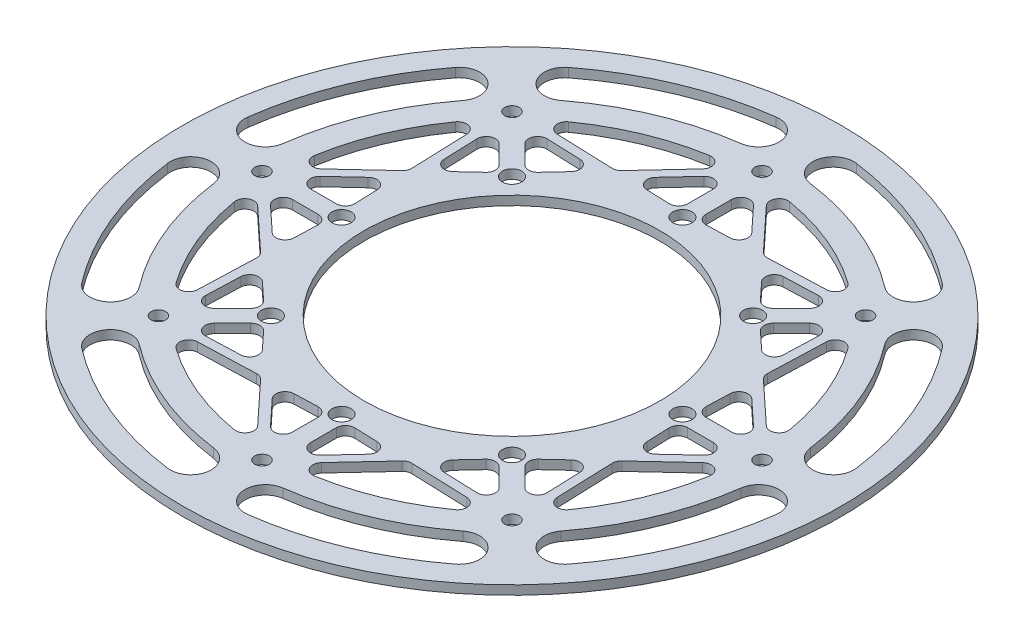
SolidWorks part; units mm, degrees
material "哈碳纤"
ref_plane "前视基准面" through (0, 0, 0) normal (0, 0, 1) x (1, 0, 0)
ref_plane "上视基准面" through (0, 0, 0) normal (0, 1, 0) x (1, 0, 0)
ref_plane "右视基准面" through (0, 0, 0) normal (1, 0, 0) x (0, 0, -1)
other "Configuration Table"
sketch "草图1" plane through (0, 0, 0) normal (0, 1, 0) x (1, 0, 0)
  line L0 (0, -1000) -> (0, 49000) construction
  line L1 (-38.352, 49.9813) -> (0, 0) construction
  line L2 (0, 0) -> (-8.2232, 62.461) construction
  line L3 (-24.1091, 58.2044) -> (0, 0) construction
  circle A0 centre (0, 0) radius 32.5
  circle A1 centre (0, 0) radius 72.5
  circle A2 centre (0, 0) radius 55 construction
  circle A3 centre (0, 55) radius 1.6
  circle A4 centre (38.8909, 38.8909) radius 1.6
  circle A5 centre (55, 0) radius 1.6
  circle A6 centre (38.8909, -38.8909) radius 1.6
  circle A7 centre (0, -55) radius 1.6
  circle A8 centre (-38.8909, -38.8909) radius 1.6
  circle A9 centre (-55, 0) radius 1.6
  circle A10 centre (-38.8909, 38.8909) radius 1.6
  circle A11 centre (0, 0) radius 37.5 construction
  circle A12 centre (0, 37.5) radius 2.1
  circle A13 centre (26.5165, 26.5165) radius 2.1
  circle A14 centre (37.5, 0) radius 2.1
  circle A15 centre (26.5165, -26.5165) radius 2.1
  circle A16 centre (0, -37.5) radius 2.1
  circle A17 centre (-26.5165, -26.5165) radius 2.1
  circle A18 centre (-37.5, 0) radius 2.1
  circle A19 centre (-26.5165, 26.5165) radius 2.1
  arc A20 (-38.352, 49.9813) -> (-8.2232, 62.461) centre (0, 0) cw construction
  arc A21 (-8.8105, 66.9225) -> (-41.0914, 53.5514) centre (0, 0) ccw
  arc A22 (-7.6358, 57.9995) -> (-35.6125, 46.4112) centre (0, 0) ccw
  arc A23 (-7.6358, 57.9995) -> (-8.8105, 66.9225) centre (-8.2232, 62.461) ccw
  arc A24 (-41.0914, 53.5514) -> (-35.6125, 46.4112) centre (-38.352, 49.9813) ccw
  arc A25 (8.2232, 62.461) -> (38.352, 49.9813) centre (0, 0) cw construction
  arc A26 (41.0914, 53.5514) -> (8.8105, 66.9225) centre (0, 0) ccw
  arc A27 (35.6125, 46.4112) -> (7.6358, 57.9995) centre (0, 0) ccw
  arc A28 (35.6125, 46.4112) -> (41.0914, 53.5514) centre (38.352, 49.9813) ccw
  arc A29 (8.8105, 66.9225) -> (7.6358, 57.9995) centre (8.2232, 62.461) ccw
  arc A30 (49.9813, 38.352) -> (62.461, 8.2232) centre (0, 0) cw construction
  arc A31 (66.9225, 8.8105) -> (53.5514, 41.0914) centre (0, 0) ccw
  arc A32 (57.9995, 7.6358) -> (46.4112, 35.6125) centre (0, 0) ccw
  arc A33 (57.9995, 7.6358) -> (66.9225, 8.8105) centre (62.461, 8.2232) ccw
  arc A34 (53.5514, 41.0914) -> (46.4112, 35.6125) centre (49.9813, 38.352) ccw
  arc A35 (62.461, -8.2232) -> (49.9813, -38.352) centre (0, 0) cw construction
  arc A36 (53.5514, -41.0914) -> (66.9225, -8.8105) centre (0, 0) ccw
  arc A37 (46.4112, -35.6125) -> (57.9995, -7.6358) centre (0, 0) ccw
  arc A38 (46.4112, -35.6125) -> (53.5514, -41.0914) centre (49.9813, -38.352) ccw
  arc A39 (66.9225, -8.8105) -> (57.9995, -7.6358) centre (62.461, -8.2232) ccw
  arc A40 (38.352, -49.9813) -> (8.2232, -62.461) centre (0, 0) cw construction
  arc A41 (8.8105, -66.9225) -> (41.0914, -53.5514) centre (0, 0) ccw
  arc A42 (7.6358, -57.9995) -> (35.6125, -46.4112) centre (0, 0) ccw
  arc A43 (7.6358, -57.9995) -> (8.8105, -66.9225) centre (8.2232, -62.461) ccw
  arc A44 (41.0914, -53.5514) -> (35.6125, -46.4112) centre (38.352, -49.9813) ccw
  arc A45 (-8.2232, -62.461) -> (-38.352, -49.9813) centre (0, 0) cw construction
  arc A46 (-41.0914, -53.5514) -> (-8.8105, -66.9225) centre (0, 0) ccw
  arc A47 (-35.6125, -46.4112) -> (-7.6358, -57.9995) centre (0, 0) ccw
  arc A48 (-35.6125, -46.4112) -> (-41.0914, -53.5514) centre (-38.352, -49.9813) ccw
  arc A49 (-8.8105, -66.9225) -> (-7.6358, -57.9995) centre (-8.2232, -62.461) ccw
  arc A50 (-49.9813, -38.352) -> (-62.461, -8.2232) centre (0, 0) cw construction
  arc A51 (-66.9225, -8.8105) -> (-53.5514, -41.0914) centre (0, 0) ccw
  arc A52 (-57.9995, -7.6358) -> (-46.4112, -35.6125) centre (0, 0) ccw
  arc A53 (-57.9995, -7.6358) -> (-66.9225, -8.8105) centre (-62.461, -8.2232) ccw
  arc A54 (-53.5514, -41.0914) -> (-46.4112, -35.6125) centre (-49.9813, -38.352) ccw
  arc A55 (-62.461, 8.2232) -> (-49.9813, 38.352) centre (0, 0) cw construction
  arc A56 (-53.5514, 41.0914) -> (-66.9225, 8.8105) centre (0, 0) ccw
  arc A57 (-46.4112, 35.6125) -> (-57.9995, 7.6358) centre (0, 0) ccw
  arc A58 (-46.4112, 35.6125) -> (-53.5514, 41.0914) centre (-49.9813, 38.352) ccw
  arc A59 (-66.9225, 8.8105) -> (-57.9995, 7.6358) centre (-62.461, 8.2232) ccw
  point P25 (0, 0)
  point P43 (0, 0)
  point P44 (-24.1091, 58.2044)
  point P56 (24.1091, 58.2044)
  point P63 (58.2044, 24.1091)
  point P70 (58.2044, -24.1091)
  point P77 (24.1091, -58.2044)
  point P84 (-24.1091, -58.2044)
  point P89 (0, 0)
  point P90 (-58.2044, -24.1091)
  point P97 (-58.2044, 24.1091)
  dimension "D1" = 65
  dimension "D2" = 145
  dimension "D3" = 110
  dimension "D4" = 3.2
  dimension "D6" = 75
  dimension "D7" = 4.2
  dimension "D9" = 9
  dimension "D10" = 63
  dimension "D11" = 30
  dimension "D13" = 22.5
  dimension "D5" = 8
  dimension "D8" = 8
  dimension "D12" = 8
extrude "凸台-拉伸1" add sketch "草图1" along normal blind 2
sketch "草图2" plane through (0, 2, 0) normal (0, 1, 0) x (1, 0, 0)
  line L0 (0, 55) -> (26.5165, 26.5165) construction
  line L1 (0, 37.5) -> (38.8909, 38.8909) construction
  line L2 (0, 55) -> (0, 37.5)
  line L3 (26.5165, 26.5165) -> (38.8909, 38.8909)
  line L4 (1.3824, 54.9826) -> (27.2241, 27.2241)
  line L5 (0, 38.5006) -> (37.9011, 39.8561)
  line L6 (0, 53.5324) -> (20.7675, 31.2244)
  line L7 (7.3941, 36.7638) -> (37.8531, 37.8531)
  line L8 (0.0357, 36.5006) -> (38.9266, 37.8915) construction
  line L9 (-0.7319, 54.3186) -> (25.7846, 25.8351) construction
  line L10 (-0.0357, 38.4994) -> (38.8551, 39.8902) construction
  line L11 (0.7319, 55.6814) -> (27.2484, 27.1979) construction
  line L12 (-1, 55) -> (-1, 37.5)
  line L13 (27.2236, 25.8094) -> (39.598, 38.1838)
  line L14 (2, 55) -> (2, 37.5)
  line L15 (25.1023, 27.9307) -> (37.4767, 40.3051)
  arc A0 (38.8909, 38.8909) -> (0, 55) centre (0, 0) ccw
  arc A1 (26.5165, 26.5165) -> (0, 37.5) centre (0, 0) ccw
  arc A2 (39.598, 39.598) -> (0, 56) centre (0, 0) ccw
  arc A3 (37.4767, 37.4767) -> (0, 53) centre (0, 0) ccw
  circle M13 centre (0, 37.5) radius 2.1
  circle M17 centre (26.5165, 26.5165) radius 2.1
  dimension "D1" = 1
  dimension "D2" = 1
  dimension "D3" = 1
  dimension "D4" = 2
  dimension "D5" = 1
  dimension "D6" = 2
extrude "切除-拉伸1" cut sketch "草图2" against normal through all both and the other way through all contours L6 L14 L5 M13 | L5 A3 L4 | L15 L7 L4 M17
fillet "圆角1" radius 2 9 edges at (13.5428, 1, -38.985) (2, 1, -38.5722) (3.3254, 1, -52.8956) (35.0514, 1, -39.7542) (16.1873, 1, -39.0796) (34.9198, 1, -37.7482) (25.8604, 1, -28.6889) (17.9903, 1, -37.1428) (2, 1, -51.384)
pattern_circular "阵列(圆周)1" count 8 over 360 about axis through (0, 0, 0) along (0, 1, 0) of "切除-拉伸1", "圆角1"
